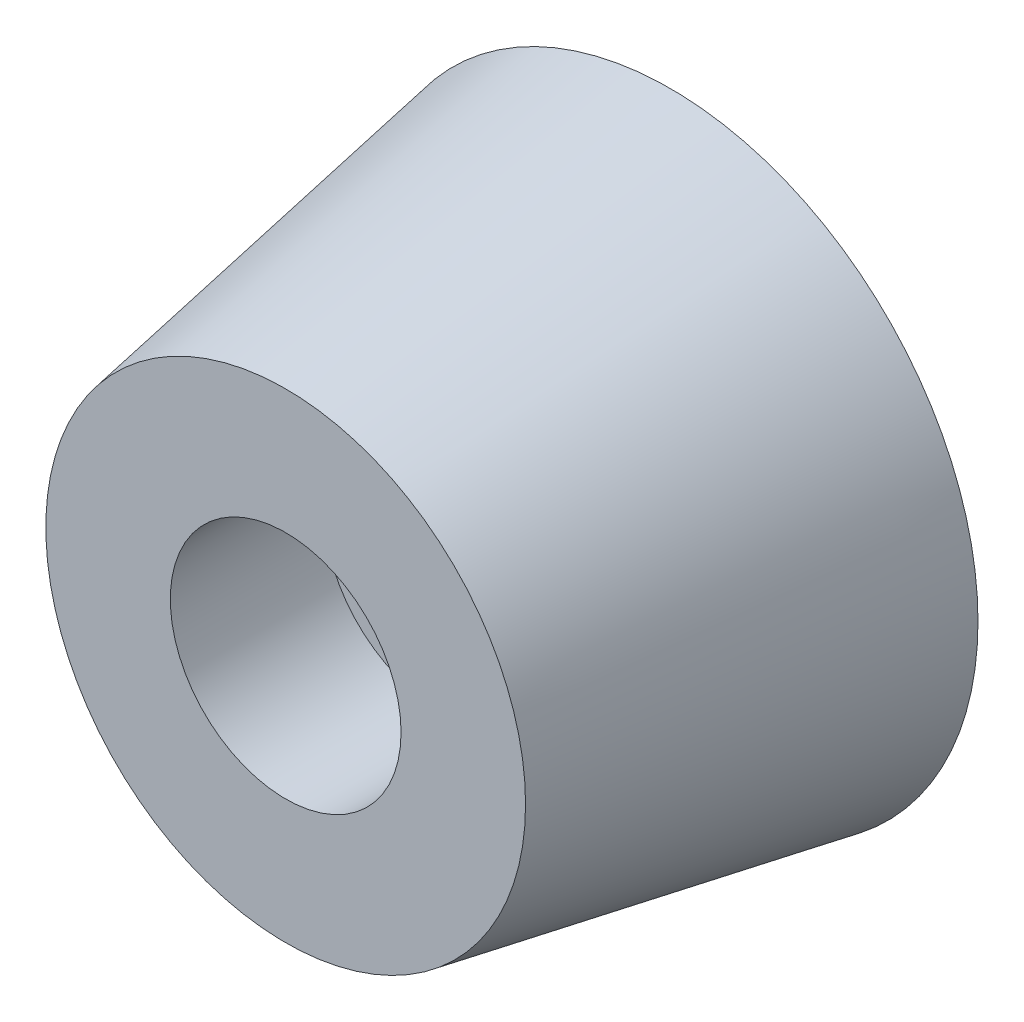
from build123d import *

# Parameters (mm, degrees)
SKETCH_1_R                = 8
EXTRUDE_1_DEPTH           = 10
EXTRUDE_1_TAPER           = 10
HOLE_WIZARD_1_D           = 3.4
HOLE_WIZARD_1_CBORE_D     = 6
HOLE_WIZARD_1_CBORE_DEPTH = 4


with BuildPart() as part:
    # 草图1 → 凸台-拉伸1 (new body)
    with BuildSketch(Plane.XY):
        Circle(SKETCH_1_R)
    extrude(amount=EXTRUDE_1_DEPTH, taper=EXTRUDE_1_TAPER)

    # 打孔尺寸(%根据)内六角圆柱头螺钉的类型1 (through all)
    with Locations(Plane.XY.offset(10)):
        with Locations((0, 0)):
            CounterBoreHole(HOLE_WIZARD_1_D / 2, HOLE_WIZARD_1_CBORE_D / 2, HOLE_WIZARD_1_CBORE_DEPTH)


solid = part.part
